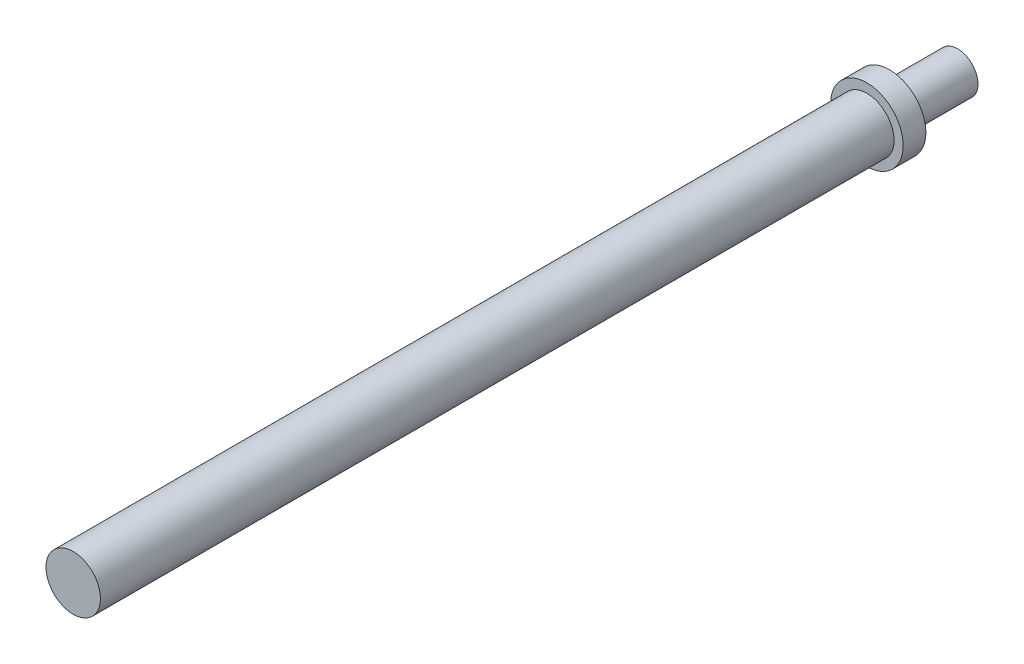
from build123d import *

# Parameters (mm, degrees)
SKETCH_1_R      = 4.5
EXTRUDE_1_DEPTH = 15
SKETCH_2_R      = 6
EXTRUDE_2_DEPTH = 180
SKETCH_3_R      = 8
EXTRUDE_3_DEPTH = 5


with BuildPart() as part:
    # 草图1 → 凸台-拉伸1 (new body)
    with BuildSketch(Plane.XY):
        Circle(SKETCH_1_R)
    extrude(amount=EXTRUDE_1_DEPTH)

    # 草图2 → 凸台-拉伸2 (add)
    with BuildSketch(Plane.XY.offset(15)):
        with Locations(Location((0, 0, 0), (0, 0, 180))):
            Circle(SKETCH_2_R)
    extrude(amount=EXTRUDE_2_DEPTH)

    # 草图3 → 凸台-拉伸3 (add)
    with BuildSketch(Plane(origin=(0, 0, 15), x_dir=(-1, 0, 0), z_dir=(0, 0, -1))):
        Circle(SKETCH_3_R)
    extrude(amount=-EXTRUDE_3_DEPTH)


solid = part.part
